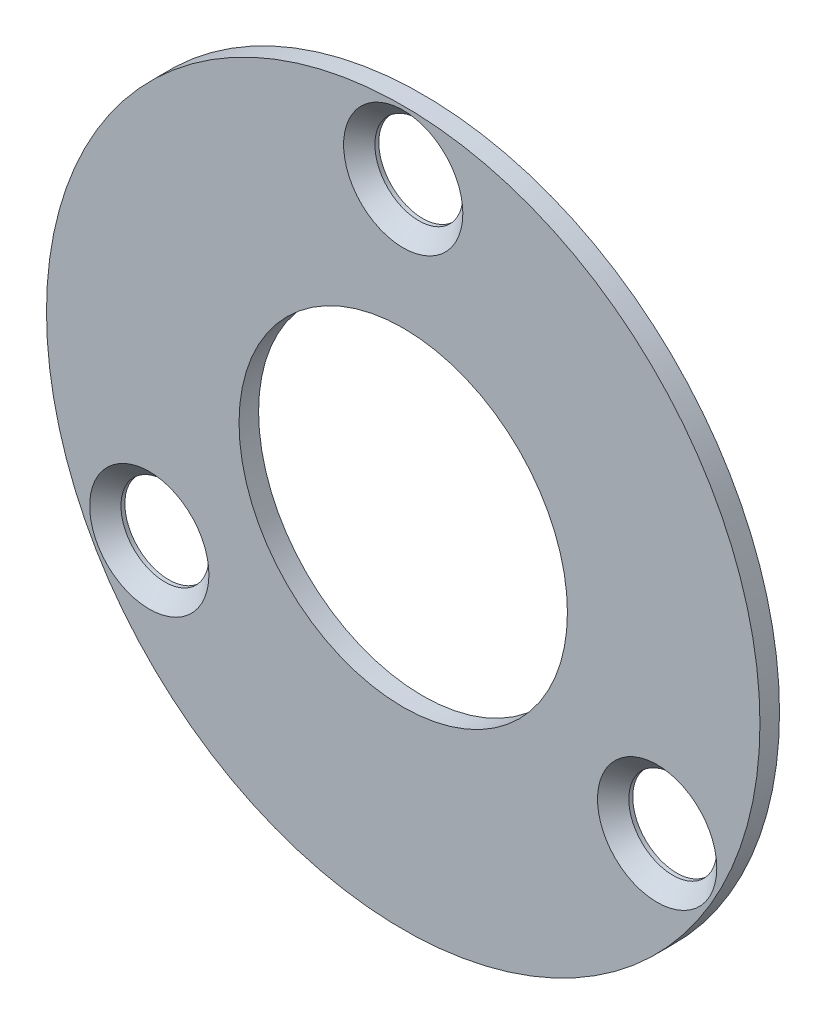
from build123d import *

# Parameters (mm, degrees)
SKETCH_1_R      = 18.25
SKETCH_1_R_2    = 8.4
SKETCH_1_R_3    = 2.25
EXTRUDE_1_DEPTH = 1
CHAMFER_1_SIZE  = 0.8


with BuildPart() as part:
    # 草图1 → 凸台-拉伸1 (new body)
    with BuildSketch(Plane.XY):
        Circle(SKETCH_1_R)
        Circle(SKETCH_1_R_2, mode=Mode.SUBTRACT)
        with Locations((0, 15)):
            Circle(SKETCH_1_R_3, mode=Mode.SUBTRACT)
        with Locations((12.990381057, -7.5)):
            Circle(SKETCH_1_R_3, mode=Mode.SUBTRACT)
        with Locations((-12.990381057, -7.5)):
            Circle(SKETCH_1_R_3, mode=Mode.SUBTRACT)
    extrude(amount=EXTRUDE_1_DEPTH)

    # 倒角1
    chamfer_1_edges = [part.edges().sort_by_distance(p)[0] for p in [
        (10.740381057, -7.5, 1),
        (-15.240381057, -7.5, 1),
        (-2.25, 15, 1),
    ]]
    chamfer(chamfer_1_edges, length=CHAMFER_1_SIZE)


solid = part.part
